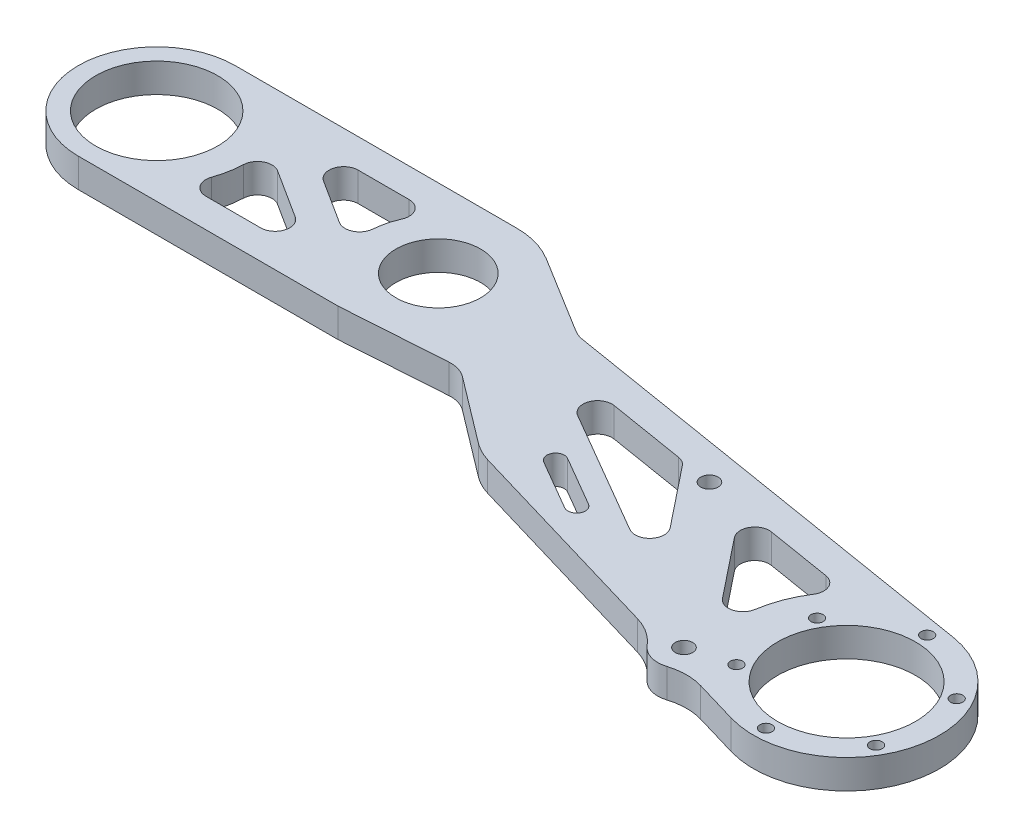
SolidWorks part; units mm, degrees
material "哈碳纤"
ref_plane "前视基准面" through (0, 0, 0) normal (0, 0, 1) x (1, 0, 0)
ref_plane "上视基准面" through (0, 0, 0) normal (0, 1, 0) x (1, 0, 0)
ref_plane "右视基准面" through (0, 0, 0) normal (1, 0, 0) x (0, 0, -1)
other "Configuration Table"
sketch "草图1" plane through (0, 0, 0) normal (0, 1, 0) x (1, 0, 0)
  line L0 (96.9499, 0) -> (288.9656, -51.4505) construction
  line L1 (0, 0) -> (96.9499, 0) construction
  line L2 (0, 27) -> (96.9499, 27)
  line L3 (0, -27) -> (90.1598, -27)
  line L5 (95.8204, -27.8178) -> (241.9443, -70.9388)
  line L6 (288.9656, -51.4505) -> (250.7853, -69.2542) construction
  line L7 (257.2952, -75.4688) -> (279.9085, -82.142)
  line L8 (96.9499, 0) -> (143.1046, 14.9966) construction
  line L10 (141.4885, 5.1281) -> (294.1373, -19.8711)
  line L11 (111.1286, 22.9775) -> (137.8532, 6.4864)
  arc A0 (0, 27) -> (0, -27) centre (0, 0) ccw
  circle A1 centre (0, 0) radius 21
  circle A2 centre (96.9499, 0) radius 14.575
  arc A3 (111.1286, 22.9775) -> (96.9499, 27) centre (96.9499, 0) ccw
  circle A4 centre (288.9656, -51.4505) radius 23.75
  circle A5 centre (288.9656, -51.4505) radius 27.75 construction
  circle A6 centre (288.9656, -23.7005) radius 2.1
  circle A7 centre (312.9978, -37.5755) radius 2.1
  circle A8 centre (312.9978, -65.3255) radius 2.1
  circle A9 centre (288.9656, -79.2005) radius 2.1
  circle A10 centre (264.9334, -65.3255) radius 2.1
  circle A11 centre (264.9334, -37.5755) radius 2.1
  arc A12 (279.9085, -82.142) -> (294.1373, -19.8711) centre (288.9656, -51.4505) ccw
  circle A13 centre (250.7853, -69.2542) radius 3
  arc A14 (241.9443, -70.9388) -> (257.2952, -75.4688) centre (250.7853, -69.2542) ccw
  arc A15 (137.8532, 6.4864) -> (141.4885, 5.1281) centre (143.1046, 14.9966) ccw
  arc A17 (95.8204, -27.8178) -> (90.1598, -27) centre (90.1598, -47) ccw
  dimension "D1" = 54
  dimension "D2" = 42
  dimension "D3" = 29.15
  dimension "D5" = 54
  dimension "D6" = 47.5
  dimension "D9" = 55.5
  dimension "D10" = 4.2
  dimension "D12" = 64
  dimension "D15" = 6
  dimension "D16" = 18
  dimension "D19" = 20
  dimension "D20" = 20
  dimension "D4" = 96.9499
  dimension "D7" = 198.7893
  dimension "D8" = 165
  dimension "D13" = 40
  dimension "D14" = 42.1273
  dimension "D17" = 48.53
  dimension "D18" = 33
  dimension "D11" = 6
extrude "凸台-拉伸1" add sketch "草图1" along normal blind 10
sketch "草图3" plane through (0, 10, 0) normal (0, 1, 0) x (1, 0, 0)
  line L0 (243.7048, -111.254) -> (131.8731, -26.617)
  line L1 (75.1615, -68.1744) -> (121.6206, -24.8506) construction
  line L2 (0, 0) -> (96.9499, 0) construction
  line L3 (95.8204, -27.8178) -> (241.9443, -70.9388) construction
  line L5 (88.8248, -27.0446) -> (125.1708, -24.6131)
  line L6 (88.8248, -27.0446) -> (243.7048, -111.254)
  arc A0 (131.8731, -26.617) -> (125.1708, -24.6131) centre (125.8383, -34.5908) ccw
  circle A1 centre (288.9656, -51.4505) radius 75 construction
  arc A3 (95.8204, -27.8178) -> (90.1598, -27) centre (90.1598, -47) ccw construction
  dimension "D1" = 150
  dimension "D5" = 10
  dimension "D2" = 43
  dimension "D3" = 2
  dimension "D4" = 35
extrude "切除-拉伸1" cut sketch "草图3" against normal blind 10
fillet "圆角1" radius 20 3 edges at (157.5159, 5, 46.024) (257.2952, 5, 75.4688) (241.9443, 5, 70.9388)
sketch "草图4" plane through (0, 10, 0) normal (0, 1, 0) x (1, 0, 0)
  line L0 (79.2036, 17) -> (25.923, 17)
  line L1 (25.923, -17) -> (79.2036, -17)
  line L7 (132.6019, -2.0237) -> (105.8772, 14.4673) construction
  line L8 (131.8731, -26.617) -> (154.6065, -43.8221)
  line L9 (161.0154, -47.0567) -> (234.1747, -68.646)
  line L11 (294.1373, -19.8711) -> (141.4885, 5.1281)
  line L12 (137.8532, 6.4864) -> (111.1286, 22.9775)
  line L13 (96.9499, 27) -> (0, 27)
  line L14 (0, -27) -> (89.4915, -27)
  line L15 (89.4915, -27) -> (125.1708, -24.6131)
  line L20 (137.8532, 6.4864) -> (111.1286, 22.9775) construction
  line L24 (25.923, 17) -> (79.2036, -17) construction
  line L25 (29.7813, 8.6066) -> (69.9088, -17)
  line L26 (35.2178, 17) -> (73.5309, -7.4488)
  line L27 (96.9499, 27) -> (0, 27) construction
  line L28 (0, -27) -> (89.4915, -27) construction
  line L29 (0, -17) -> (89.1574, -17) construction
  line L30 (96.9499, 17) -> (0, 17) construction
  line L31 (23.2333, 12.7851) -> (76.5139, -21.2149) construction
  line L32 (28.6126, 21.2149) -> (81.8932, -12.7851) construction
  line L33 (89.4915, -27) -> (125.1708, -24.6131) construction
  line L34 (137.9079, -18.6432) -> (160.6412, -35.8483) construction
  line L35 (163.9983, -37.5094) -> (208.6493, -60.5435) construction
  line L36 (278.7043, -72.3825) -> (280.5631, -71.7827) construction
  line L37 (292.5211, -29.7397) -> (139.8723, -4.7405) construction
  line L38 (131.8731, -26.617) -> (154.6065, -43.8221) construction
  line L39 (160.1705, -46.7869) -> (210.3293, -72.6624) construction
  line L40 (273.006, -84.7293) -> (280.5008, -82.3106) construction
  line L41 (294.1373, -19.8711) -> (141.4885, 5.1281) construction
  line L42 (89.1574, -17) -> (124.5033, -14.6354) construction
  line L43 (229.3437, -56.794) -> (185.7649, -2.1231)
  line L44 (294.1373, -19.8711) -> (141.4885, 5.1281) construction
  line L45 (257.9245, -66.9803) -> (209.2981, -5.9771)
  line L46 (161.0154, -47.0567) -> (234.1747, -68.646) construction
  line L47 (139.8723, -4.7405) -> (229.3437, -56.794)
  line L48 (229.3437, -56.794) -> (252.1306, -59.7117)
  line L60 (265.0648, -77.7616) -> (279.9085, -82.142)
  line L94 (282.7389, -72.5509) -> (267.8951, -68.1705)
  line L95 (139.8723, -4.7405) -> (292.5211, -29.7397)
  line L96 (237.005, -59.0549) -> (163.8457, -37.4656)
  line L97 (160.6412, -35.8483) -> (137.9079, -18.6432)
  line L98 (282.7389, -72.5509) -> (267.8951, -68.1705)
  line L99 (139.8723, -4.7405) -> (292.5211, -29.7397)
  line L100 (237.005, -59.0549) -> (229.3437, -56.794)
  circle A0 centre (96.9499, 0) radius 14.575 construction
  circle A1 centre (0, 0) radius 21 construction
  circle A2 centre (96.9499, 0) radius 14.575 construction
  circle A3 centre (0, 0) radius 21 construction
  arc A4 (79.2036, 17) -> (79.2036, -17) centre (96.9499, 0) ccw
  arc A5 (25.923, -17) -> (25.923, 17) centre (0, 0) ccw
  arc A9 (154.6065, -43.8221) -> (161.0154, -47.0567) centre (166.676, -27.8745) ccw
  arc A13 (279.9085, -82.142) -> (294.1373, -19.8711) centre (288.9656, -51.4505) ccw
  arc A14 (137.8532, 6.4864) -> (141.4885, 5.1281) centre (143.1046, 14.9966) ccw
  arc A15 (111.1286, 22.9775) -> (96.9499, 27) centre (96.9499, 0) ccw
  arc A16 (0, 27) -> (0, -27) centre (0, 0) ccw
  arc A17 (131.8731, -26.617) -> (125.1708, -24.6131) centre (125.8383, -34.5908) ccw
  circle A33 centre (0, 0) radius 31 construction
  arc A34 (0, 27) -> (0, -27) centre (0, 0) ccw construction
  circle A35 centre (0, 0) radius 21 construction
  arc A36 (0, 17) -> (0, -17) centre (0, 0) ccw construction
  circle A37 centre (96.9499, 0) radius 24.575 construction
  arc A38 (111.1286, 22.9775) -> (96.9499, 27) centre (96.9499, 0) ccw construction
  arc A39 (131.8731, -26.617) -> (125.1708, -24.6131) centre (125.8383, -34.5908) ccw construction
  arc A40 (160.6412, -35.8483) -> (163.9983, -37.5094) centre (166.676, -27.8745) ccw construction
  arc A41 (154.6065, -43.8221) -> (160.1705, -46.7869) centre (166.676, -27.8745) ccw construction
  arc A42 (247.7907, -82.699) -> (210.3293, -72.6624) centre (226.9033, -85.7305) ccw construction
  arc A43 (247.7907, -82.699) -> (258.9343, -81.3135) centre (251.7104, -68.719) ccw construction
  arc A44 (273.006, -84.7293) -> (258.9343, -81.3135) centre (265.7678, -83.8551) ccw construction
  arc A45 (280.5008, -82.3106) -> (294.1373, -19.8711) centre (288.9656, -51.4505) ccw construction
  arc A46 (137.8532, 6.4864) -> (141.4885, 5.1281) centre (143.1046, 14.9966) ccw construction
  arc A47 (254.2692, -70.9418) -> (208.6493, -60.5435) centre (226.9033, -85.7305) ccw construction
  arc A48 (254.2692, -70.9418) -> (254.2692, -70.9418) centre (254.2692, -70.9418) ccw construction
  arc A49 (278.7043, -72.3825) -> (254.2692, -70.9418) centre (265.7678, -83.8551) ccw construction
  arc A50 (280.5631, -71.7827) -> (292.5211, -29.7397) centre (288.9656, -51.4505) ccw construction
  arc A51 (132.6019, -2.0237) -> (139.8723, -4.7405) centre (143.1046, 14.9966) ccw construction
  arc A52 (137.9079, -18.6432) -> (124.5033, -14.6354) centre (125.8383, -34.5908) ccw construction
  arc A53 (105.8772, 14.4673) -> (96.9499, 17) centre (96.9499, 0) ccw construction
  arc A65 (243.8735, -75.0186) -> (234.1747, -68.646) centre (228.514, -87.8282) ccw
  arc A66 (243.8735, -75.0186) -> (253.4601, -77.8475) centre (250.7853, -69.2542) ccw
  arc A67 (265.0648, -77.7616) -> (253.4601, -77.8475) centre (259.4042, -96.9438) ccw
  arc A87 (243.8735, -75.0186) -> (253.4601, -77.8475) centre (250.7853, -69.2542) ccw construction
  circle A88 centre (288.9656, -51.4505) radius 37.75
  arc A89 (262.2477, -24.7818) -> (254.7102, -67.3133) centre (288.9656, -51.4505) ccw
  arc A91 (251.1231, -68.1094) -> (237.005, -59.0549) centre (228.514, -87.8282) ccw
  arc A92 (267.8951, -68.1705) -> (251.1231, -68.1094) centre (259.4042, -96.9438) ccw
  arc A93 (282.7389, -72.5509) -> (292.5211, -29.7397) centre (288.9656, -51.4505) ccw
  arc A94 (160.6412, -35.8483) -> (163.8457, -37.4656) centre (166.676, -27.8745) ccw
  arc A95 (251.1231, -68.1094) -> (237.005, -59.0549) centre (228.514, -87.8282) ccw
  arc A96 (267.8951, -68.1705) -> (251.1231, -68.1094) centre (259.4042, -96.9438) ccw
  arc A97 (282.7389, -72.5509) -> (292.5211, -29.7397) centre (288.9656, -51.4505) ccw
  point P88 (255.6706, -96.4387)
  point P91 (221.1426, -86.2384)
  dimension "D3" = 10
  dimension "D4" = 5
  dimension "D6" = 16
  dimension "D8" = 14
  dimension "D9" = 35
  dimension "D1" = 0
  dimension "D2" = 10
  dimension "D5" = 5
  dimension "D7" = 10
extrude "切除-拉伸2" cut sketch "草图4" against normal blind 10
fillet "圆角2" radius 5 12 edges at (29.7813, 5, -8.6066) (69.9088, 5, 17) (25.923, 5, 17) (252.1306, 5, 59.7117) (218.5882, 5, 17.6317) (73.5309, 5, 7.4488) (35.2178, 5, -17) (79.2036, 5, -17) (195.0549, 5, 13.7777) (262.2477, 5, 24.7818) (139.8723, 5, 4.7405) (229.3437, 5, 56.794)
sketch "草图5" plane through (0, 10, 0) normal (0, 1, 0) x (1, 0, 0)
  line L0 (294.1373, -19.8711) -> (141.4885, 5.1281) construction
  line L5 (137.8532, 6.4864) -> (111.1286, 22.9775) construction
  circle A0 centre (205.8459, -15.5449) radius 3
  circle A1 centre (96.9499, 0) radius 14.575 construction
  circle A2 centre (125.8459, 2.1452) radius 3 construction
  dimension "D1" = 6
  dimension "D3" = 110
  dimension "D4" = 6
  dimension "D2" = 10
  dimension "D5" = 10
  dimension "D6" = 80
extrude "切除-拉伸3" cut sketch "草图5" against normal blind 10
sketch "草图6" plane through (0, 0, 0) normal (0, -1, 0) x (1, 0, 0)
  line L1 (220.2856, 26.5449) -> (165.876, 23.407) construction
  line L2 (165.876, 23.407) -> (164.8396, 41.3771) construction
  line L3 (164.8396, 41.3771) -> (219.2492, 44.5151) construction
  line L4 (219.2492, 44.5151) -> (220.2856, 26.5449) construction
  line L6 (294.1373, 19.8711) -> (141.4885, -5.1281) construction
  circle A0 centre (288.9656, 51.4505) radius 23.75 construction
  circle A1 centre (164.8396, 41.3771) radius 1.1
  circle A2 centre (219.2492, 44.5151) radius 1.1
  circle A3 centre (165.876, 23.407) radius 1.1
  circle A4 centre (220.2856, 26.5449) radius 1.1
  circle A5 centre (205.8459, 15.5449) radius 3 construction
  dimension "D5" = 2.2
  dimension "D1" = 18
  dimension "D2" = 54.5
  dimension "D3" = 70
  dimension "D4" = 6
  dimension "D6" = 11
extrude "切除-拉伸4" [suppressed] cut sketch "草图6" against normal blind 10
sketch "草图7" plane through (0, 0, 0) normal (0, -1, 0) x (1, 0, 0)
  line L0 (172.8297, 35.484) -> (190.1169, 45.5415) construction
  line L1 (171.3211, 38.0771) -> (188.6082, 48.1346)
  line L2 (174.3383, 32.8909) -> (191.6255, 42.9484)
  line L3 (163.3166, 18.3801) -> (206.307, 43.3915) construction
  arc A0 (171.3211, 38.0771) -> (174.3383, 32.8909) centre (172.8297, 35.484) ccw
  arc A1 (191.6255, 42.9484) -> (188.6082, 48.1346) centre (190.1169, 45.5415) ccw
  point P2 (181.4733, 40.5128)
  dimension "D1" = 10
  dimension "D2" = 6
  dimension "D3" = 20
  dimension "D4" = 25
extrude "切除-拉伸5" cut sketch "草图7" against normal blind 10
